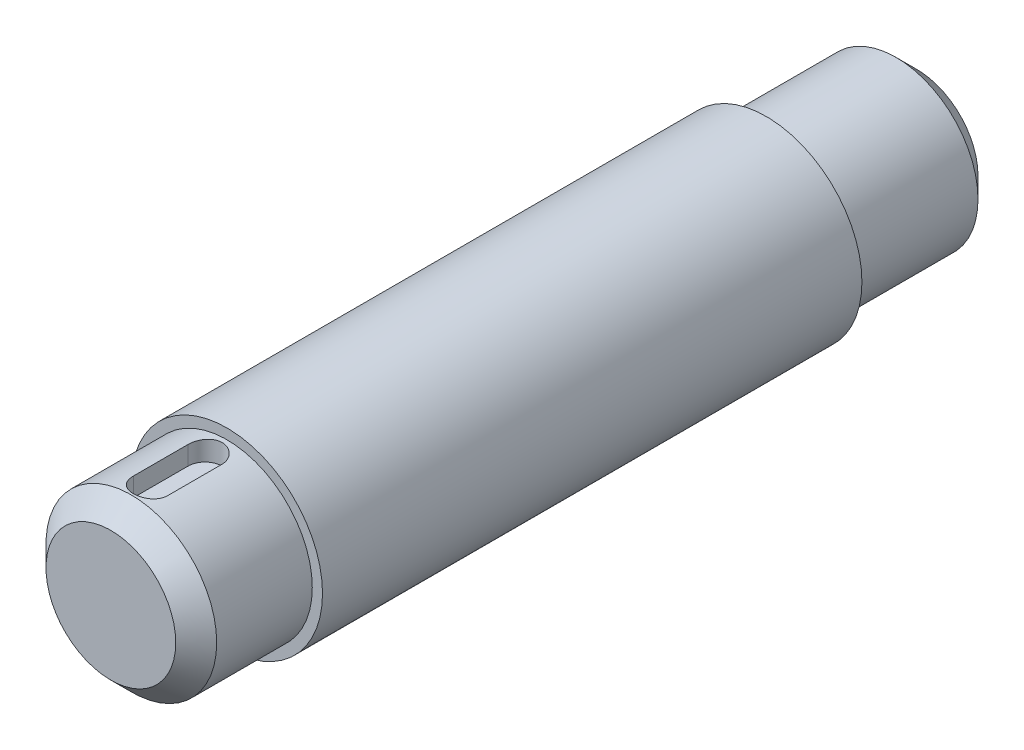
from build123d import *

# Parameters (mm, degrees)
SKETCH1_R           = 12
BOSS_EXTRUDE1_DEPTH = 22
SKETCH2_R           = 14
BOSS_EXTRUDE2_DEPTH = 96
CUT_EXTRUDE1_START  = -66
SKETCH3_R           = 14
SKETCH3_R_2         = 12.5
CUT_EXTRUDE1_DEPTH  = 66
CHAMFER1_SIZE       = 3
MOVE_FACE1_BY       = 49
CUT_EXTRUDE2_DEPTH  = 3


with BuildPart() as part:
    # Sketch1 → Boss-Extrude1 (new body)
    with BuildSketch(Plane.XY):
        Circle(SKETCH1_R)
    extrude(amount=-BOSS_EXTRUDE1_DEPTH)

    # Sketch2 → Boss-Extrude2 (add)
    with BuildSketch(Plane.XY):
        Circle(SKETCH2_R)
    extrude(amount=BOSS_EXTRUDE2_DEPTH)

    # Sketch3 → Cut-Extrude1 (cut)
    with BuildSketch(Plane.XY.offset(96).offset(CUT_EXTRUDE1_START)):
        Circle(SKETCH3_R)
        Circle(SKETCH3_R_2, mode=Mode.SUBTRACT)
    extrude(amount=CUT_EXTRUDE1_DEPTH, mode=Mode.SUBTRACT)

    # Chamfer1
    chamfer1_edges = [part.edges().sort_by_distance(p)[0] for p in [
        (-12.5, 0, 96),
        (-12, 0, -22),
    ]]
    chamfer(chamfer1_edges, length=CHAMFER1_SIZE)

    # Move Face1: a face moved outward by 49.0
    extrude(part.faces().sort_by_distance((-7, -11.2, 30))[0], amount=MOVE_FACE1_BY, dir=(0, 0, 1))

    # Sketch4 → Cut-Extrude2 (cut)
    with BuildSketch(Plane(origin=(0, 12.5, 0), x_dir=(1, 0, 0), z_dir=(0, 1, 0))):
        with BuildLine():
            Line((-2.5, -90.2), (-2.5, -82.2))
            ThreePointArc((-2.5, -82.2), (0, -79.7), (2.5, -82.2))
            Line((2.5, -82.2), (2.5, -90.2))
            ThreePointArc((2.5, -90.2), (0, -92.7), (-2.5, -90.2))
        make_face()
    extrude(amount=-CUT_EXTRUDE2_DEPTH, mode=Mode.SUBTRACT)


solid = part.part
